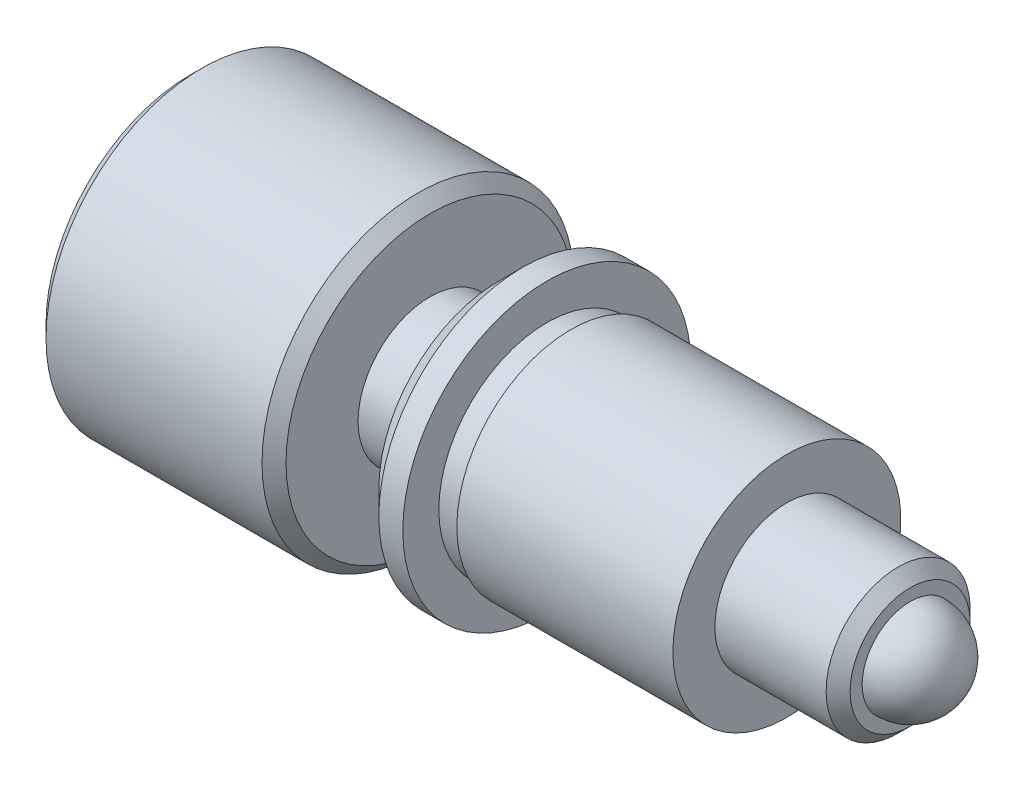
SolidWorks part; units mm, degrees
ref_plane "Front Plane" through (0, 0, 0) normal (0, 0, 1) x (1, 0, 0)
ref_plane "Top Plane" through (0, 0, 0) normal (0, 1, 0) x (1, 0, 0)
ref_plane "Right Plane" through (0, 0, 0) normal (1, 0, 0) x (0, 0, -1)
sketch "Sketch1" plane through (0, 0, 0) normal (0, 1, 0) x (1, 0, 0)
  line L0 (-122.4327, 0) -> (5999.2013, 0) construction
  line L1 (-15.5459, 0) -> (-15.5459, 6)
  line L2 (-15.0459, 6.5) -> (-6.0459, 6.5)
  line L3 (-5.5459, 6) -> (-5.5459, 3)
  line L4 (-5.5459, 3) -> (-2.6801, 3)
  line L5 (-2.6801, 3) -> (-2.6801, 5)
  line L6 (-1.6801, 6) -> (-0.6801, 6)
  line L7 (-0.6801, 6) -> (-0.6801, 4.5)
  line L8 (-0.6801, 4.5) -> (0.3199, 4.5)
  line L9 (0.3199, 4.5) -> (0.3199, 4.75)
  line L10 (0.3199, 4.75) -> (9.3199, 4.75)
  line L11 (9.3199, 4.75) -> (9.3199, 3)
  line L12 (9.3199, 3) -> (13.9541, 3)
  line L13 (14.4541, 2.5) -> (14.4541, 2)
  line L14 (-15.5459, 6) -> (-15.0459, 6.5)
  line L15 (-6.0459, 6.5) -> (-5.5459, 6)
  line L16 (-2.6801, 5) -> (-1.6801, 6)
  line L17 (13.9541, 3) -> (14.4541, 2.5)
  line L19 (-15.5459, 0) -> (16.4541, 0)
  arc A1 (16.4541, 0) -> (14.4541, 2) centre (14.4541, 0) ccw
  point P4 (-15.5459, 6.5)
  point P6 (-5.5459, 6.5)
  point P9 (-2.6801, 6)
  point P16 (14.4541, 3)
  dimension "D12" = 4
  dimension "D1" = 6.5
  dimension "D2" = 10
  dimension "D3" = 4.75
  dimension "D4" = 6
  dimension "D5" = 4.5
  dimension "D6" = 3
  dimension "D7" = 3
  dimension "D8" = 2
  dimension "D9" = 12
  dimension "D10" = 20
  dimension "D11" = 1
revolve "Revolve1" add sketch "Sketch1" angle 360 about L0
cosmetic thread "Cosmetic Thread1"
cosmetic thread "Cosmetic Thread2"
